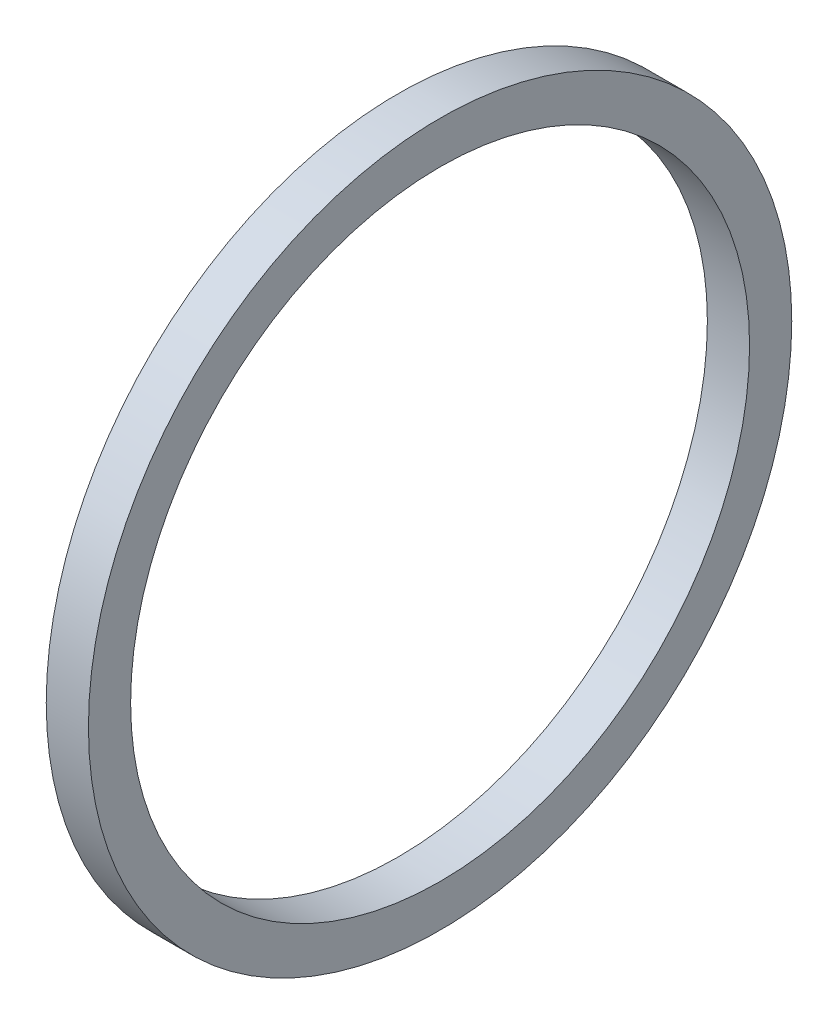
from build123d import *


with BuildPart() as part:
    # Sketch1 → Revolve1 (revolve)
    with BuildSketch(Plane.XY, mode=Mode.PRIVATE) as revolve1_sk:
        Polygon((-50, 48.55), (-50, 50), (-44, 50), (-44, 44), (-50, 44), (-50, 46), (-45.5, 46), (-45.5, 48.55), align=None)
    revolve(revolve1_sk.sketch.rotate(Axis((0, 0, 0), (-1, 0, 0)), 90), axis=Axis((0, 0, 0), (-1, 0, 0)))


solid = part.part
